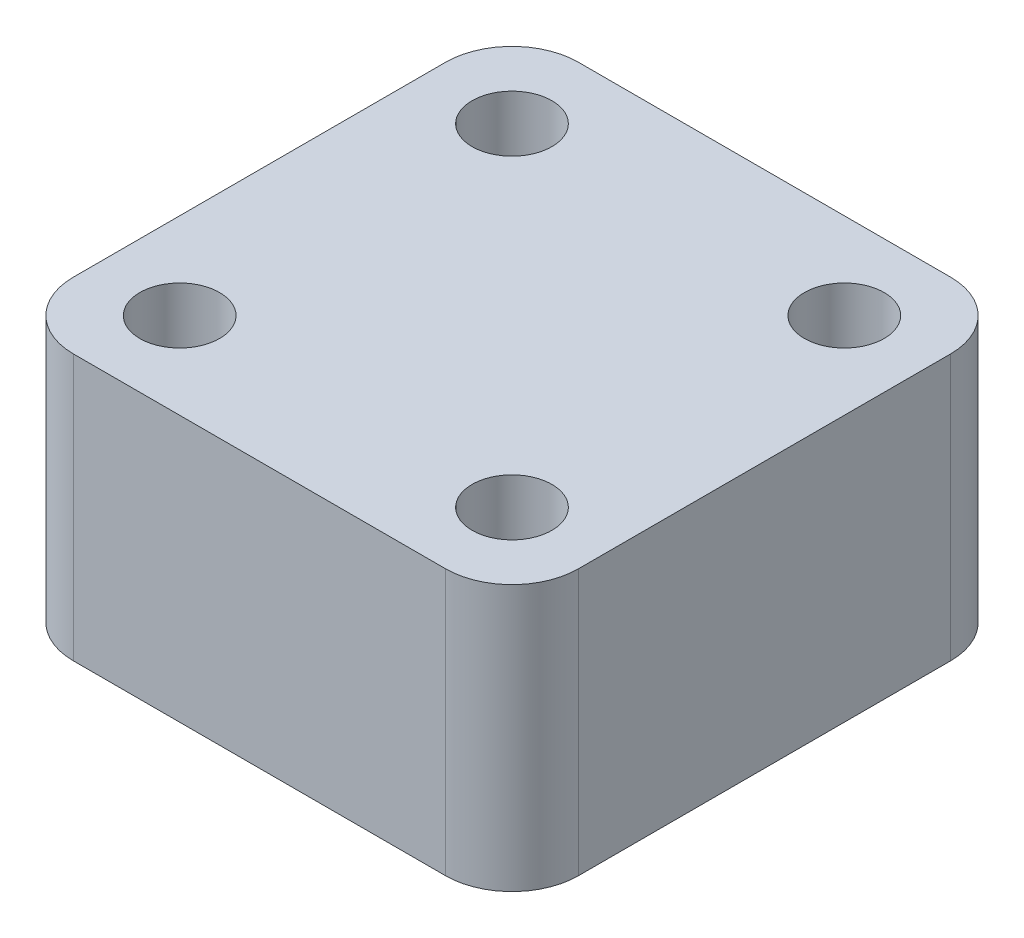
from build123d import *

# Parameters (mm, degrees)
BOSS_EXTRUDE1_DEPTH                                = 20
HOLE_SIZE_BASED_ON_SOCKET_HEAD_CAP_SCR_D           = 3.4
HOLE_SIZE_BASED_ON_SOCKET_HEAD_CAP_SCR_CBORE_D     = 6
HOLE_SIZE_BASED_ON_SOCKET_HEAD_CAP_SCR_CBORE_DEPTH = 10


with BuildPart() as part:
    # Sketch1 → Boss-Extrude1 (new body)
    with BuildSketch(Plane(origin=(0, 0, 0), x_dir=(1, 0, 0), z_dir=(0, 1, 0))):
        with BuildLine():
            Line((-14, 19), (14, 19))
            ThreePointArc((14, 19), (17.535533906, 17.535533906), (19, 14))
            Line((19, 14), (19, -14))
            ThreePointArc((19, -14), (17.535533906, -17.535533906), (14, -19))
            Line((14, -19), (-14, -19))
            ThreePointArc((-14, -19), (-17.535533906, -17.535533906), (-19, -14))
            Line((-19, -14), (-19, 14))
            ThreePointArc((-19, 14), (-17.535533906, 17.535533906), (-14, 19))
        make_face()
    extrude(amount=BOSS_EXTRUDE1_DEPTH)

    # Hole size (%based on) socket head cap screw type 1 (through all)
    with Locations(Plane(origin=(0, 20, 0), x_dir=(1, 0, 0), z_dir=(0, 1, 0))):
        with Locations((-12.5, 12.5), (12.5, 12.5), (12.5, -12.5), (-12.5, -12.5)):
            CounterBoreHole(HOLE_SIZE_BASED_ON_SOCKET_HEAD_CAP_SCR_D / 2, HOLE_SIZE_BASED_ON_SOCKET_HEAD_CAP_SCR_CBORE_D / 2, HOLE_SIZE_BASED_ON_SOCKET_HEAD_CAP_SCR_CBORE_DEPTH)


solid = part.part
